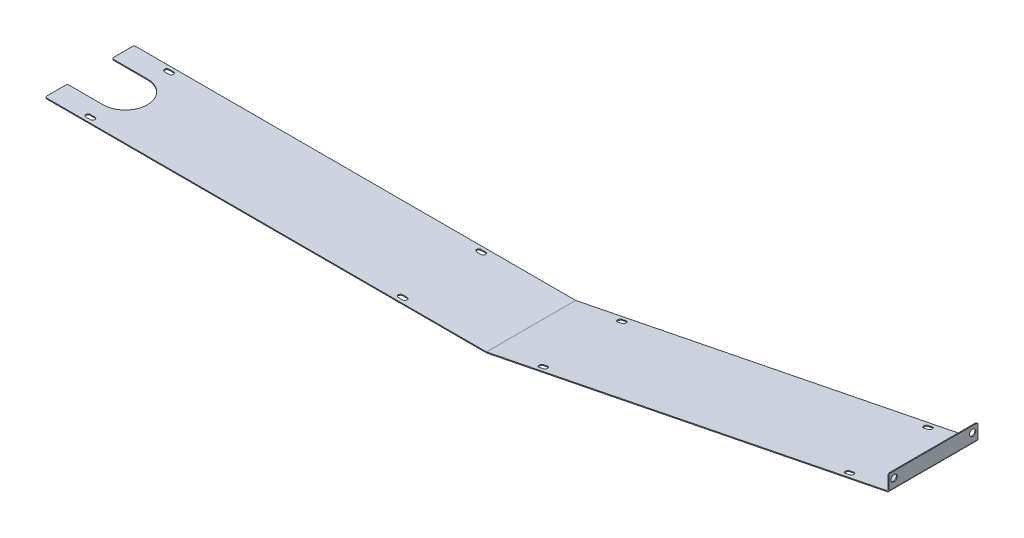
SolidWorks part; units mm, degrees
ref_plane "Front Plane" through (0, 0, 0) normal (0, 0, 1) x (1, 0, 0)
ref_plane "Top Plane" through (0, 0, 0) normal (0, 1, 0) x (1, 0, 0)
ref_plane "Right Plane" through (0, 0, 0) normal (1, 0, 0) x (0, 0, -1)
sketch "Sketch1" plane through (0, 0, 0) normal (0, 0, 1) x (1, 0, 0)
  line L0 (0, 0) -> (495, 0)
  line L1 (495, 0) -> (945, 90)
  line L2 (945, 90) -> (945, 107)
  dimension "D1" = 495
  dimension "D2" = 450
  dimension "D3" = 90
  dimension "D4" = 107
extrude "Extrude-Thin1" add sketch "Sketch1" along normal mid plane 100 thin
sketch "Sketch2" plane through (945, 0, 0) normal (-1, 0, 0) x (0, 0, 1)
  line L0 (-50, 90) -> (-50, 107) construction
  line L2 (50, 107) -> (-50, 107) construction
  circle A0 centre (-44, 100) radius 3.5
  circle A1 centre (44, 100) radius 3.5
  dimension "D1" = 7
  dimension "D2" = 88
  dimension "D3" = 6
  dimension "D4" = 7
extrude "Cut-Extrude1" cut sketch "Sketch2" against normal through all
sketch "Sketch3" plane through (0, -1, 0) normal (0, -1, 0) x (1, 0, 0)
  line L1 (42.5, 44) -> (47.5, 44) construction
  line L2 (42.5, 46.5) -> (47.5, 46.5)
  line L3 (42.5, 41.5) -> (47.5, 41.5)
  line L4 (42.5, -44) -> (47.5, -44) construction
  line L5 (42.5, -41.5) -> (47.5, -41.5)
  line L6 (42.5, -46.5) -> (47.5, -46.5)
  line L7 (392.5, -44) -> (397.5, -44) construction
  line L8 (392.5, -41.5) -> (397.5, -41.5)
  line L9 (392.5, -46.5) -> (397.5, -46.5)
  line L10 (392.5, 44) -> (397.5, 44) construction
  line L11 (392.5, 46.5) -> (397.5, 46.5)
  line L12 (392.5, 41.5) -> (397.5, 41.5)
  line L13 (0, 50) -> (0, -50) construction
  line L14 (0, 50) -> (495.099, 50) construction
  arc A4 (42.5, 46.5) -> (42.5, 41.5) centre (42.5, 44) ccw
  arc A5 (47.5, 41.5) -> (47.5, 46.5) centre (47.5, 44) ccw
  arc A6 (42.5, -41.5) -> (42.5, -46.5) centre (42.5, -44) ccw
  arc A7 (47.5, -46.5) -> (47.5, -41.5) centre (47.5, -44) ccw
  arc A8 (392.5, -41.5) -> (392.5, -46.5) centre (392.5, -44) ccw
  arc A9 (397.5, -46.5) -> (397.5, -41.5) centre (397.5, -44) ccw
  arc A10 (392.5, 46.5) -> (392.5, 41.5) centre (392.5, 44) ccw
  arc A11 (397.5, 41.5) -> (397.5, 46.5) centre (397.5, 44) ccw
  point P13 (45, 44)
  point P19 (45, -44)
  point P26 (395, -44)
  point P34 (395, 44)
  dimension "D1" = 45
  dimension "D2" = 350
  dimension "D3" = 88
  dimension "D4" = 6
  dimension "D5" = 5
  dimension "D6" = 5
extrude "Cut-Extrude2" cut sketch "Sketch3" against normal through all
sketch "Sketch4" plane through (19.0385, -95.1923, 0) normal (-0.1961, 0.9806, 0) x (0.9806, 0.1961, 0)
  line L2 (541.7992, 44) -> (546.7992, 44) construction
  line L3 (541.7992, 46.5) -> (546.7992, 46.5)
  line L4 (541.7992, 41.5) -> (546.7992, 41.5)
  line L5 (541.7992, -44) -> (546.7992, -44) construction
  line L6 (541.7992, -41.5) -> (546.7992, -41.5)
  line L7 (541.7992, -46.5) -> (546.7992, -46.5)
  line L8 (891.7992, -44) -> (896.7992, -44) construction
  line L9 (891.7992, -41.5) -> (896.7992, -41.5)
  line L10 (891.7992, -46.5) -> (896.7992, -46.5)
  line L11 (891.7992, 44) -> (896.7992, 44) construction
  line L12 (891.7992, 46.5) -> (896.7992, 46.5)
  line L13 (891.7992, 41.5) -> (896.7992, 41.5)
  line L14 (944.2992, -50) -> (944.2992, 50) construction
  line L15 (485.3874, -50) -> (944.2992, -50) construction
  arc A4 (541.7992, 46.5) -> (541.7992, 41.5) centre (541.7992, 44) ccw
  arc A5 (546.7992, 41.5) -> (546.7992, 46.5) centre (546.7992, 44) ccw
  arc A6 (541.7992, -41.5) -> (541.7992, -46.5) centre (541.7992, -44) ccw
  arc A7 (546.7992, -46.5) -> (546.7992, -41.5) centre (546.7992, -44) ccw
  arc A8 (891.7992, -41.5) -> (891.7992, -46.5) centre (891.7992, -44) ccw
  arc A9 (896.7992, -46.5) -> (896.7992, -41.5) centre (896.7992, -44) ccw
  arc A10 (891.7992, 46.5) -> (891.7992, 41.5) centre (891.7992, 44) ccw
  arc A11 (896.7992, 41.5) -> (896.7992, 46.5) centre (896.7992, 44) ccw
  point P14 (544.2992, 44)
  point P20 (544.2992, -44)
  point P27 (894.2992, -44)
  point P34 (894.2992, 44)
  dimension "D1" = 50
  dimension "D2" = 88
  dimension "D3" = 6
  dimension "D4" = 5
  dimension "D5" = 5
  dimension "D6" = 350
extrude "Cut-Extrude3" cut sketch "Sketch4" against normal through all
sketch "Sketch5" plane through (0, 0, 0) normal (0, 1, 0) x (1, 0, 0)
  line L0 (0, 0) -> (253.2768, 0) construction
  line L1 (0, -50) -> (0, 50) construction
  line L2 (0, -25) -> (40, -25)
  line L3 (0, -25) -> (0, 25)
  line L4 (0, 25) -> (40, 25)
  arc A0 (40, 25) -> (40, -25) centre (40, 0) cw
  dimension "D1" = 40
  dimension "D2" = 50
extrude "Cut-Extrude4" cut sketch "Sketch5" against normal through all
fillet "Fillet1" radius 2 10 edges at (0, -0.5, -50) (0, -0.5, 50) (495.099, -1, 0) (495, 0, 0) (946, 89.1802, 0) (945, 90, 0) (945.5, 107, 50) (945.5, 107, -50) (0, -0.5, 25) (0, -0.5, -25)
